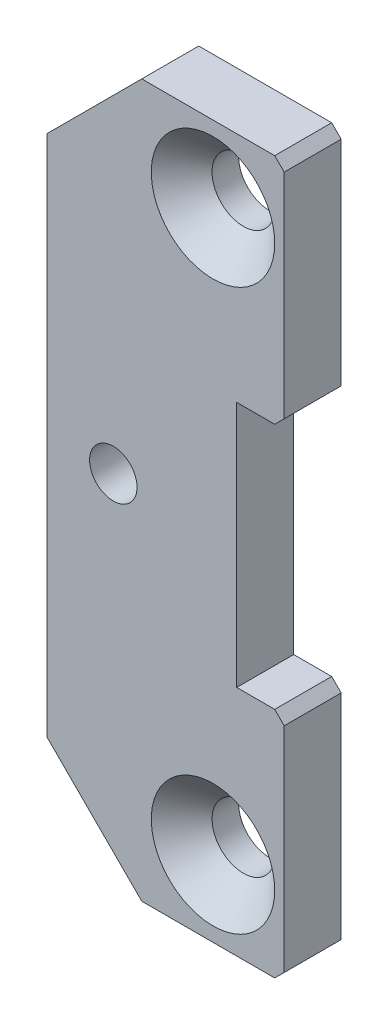
SolidWorks part; units mm, degrees
material "Q235-A"
ref_plane "Front Plane" through (0, 0, 0) normal (0, 0, 1) x (1, 0, 0)
ref_plane "Top Plane" through (0, 0, 0) normal (0, 1, 0) x (1, 0, 0)
ref_plane "Right Plane" through (0, 0, 0) normal (1, 0, 0) x (0, 0, -1)
sketch "Sketch1" plane through (0, 0, 0) normal (0, 0, 1) x (1, 0, 0)
  line L0 (0, 75) -> (0, 0)
  dimension "D2" = 75
extrude "Extrude-Thin1" add sketch "Sketch1" along normal blind 6 thin
chamfer "Chamfer1" distance 1 angle 45 2 edges at (0, 75, 3) (0, 0, 3)
hole_wizard "Hole size (per socket flat counteBLZKk head screw type)1" positions "Sketch7" profile "Sketch9" countersink size "M6" standard "GB" end condition through all
sketch "Sketch7" plane through (0, 0, 6) normal (0, 0, 1) x (1, 0, 0)
  line L1 (-25, 75) -> (-1, 75) construction
  line L4 (-25, 37.5) -> (0, 37.5) construction
  line L5 (-25, 75) -> (-25, 0) construction
  line L6 (0, 74) -> (0, 1) construction
  point P0 (-7.5, 67)
  point P2 (-7.5, 8)
  dimension "D1" = 8
  dimension "D2" = 7.5
sketch "Sketch9" plane through (-7.5, 67, 6) normal (1, 0, 0) x (0, -1, 0)
  line L0 (0, 0) -> (0, 6)
  line L1 (0, 6) -> (3.3, 6)
  line L2 (3.3, 6) -> (3.3, 3.2)
  line L3 (3.3, 3.2) -> (6.5, 0)
  line L5 (6.5, 0) -> (0, 0)
  line L6 (-3.3, 3.2) -> (-6.5, 0) construction
  line L11 (0, -6.35) -> (0, 107.95) construction
  dimension "通孔孔直径" = 6.6
  dimension "通孔孔深度" = 6
  dimension "近端锥形沉头孔直径" = 13
  dimension "近端锥形沉头孔角度" = 90
chamfer "Chamfer2" distance 10 angle 45 2 edges at (-25, 0, 3) (-25, 75, 3)
hole_wizard "M6 Tapped Hole1" positions "Sketch10" profile "Sketch11" tap size "M6" standard "GB" end condition through all
sketch "Sketch10" plane through (0, 0, 6) normal (0, 0, 1) x (1, 0, 0)
  line L0 (0, 37.5) -> (-51.0681, 37.5)
  line L1 (0, 74) -> (0, 1) construction
  line L3 (-25, 65) -> (-25, 10) construction
  point P0 (-18, 37.5)
  dimension "D1" = 7
sketch "Sketch11" plane through (-18, 37.5, 6) normal (1, 0, 0) x (0, -1, 0)
  line L0 (0, 0) -> (0, 6)
  line L1 (0, 6) -> (2.5, 6)
  line L2 (2.5, 6) -> (2.5, 0)
  line L5 (2.5, 0) -> (0, 0)
  line L11 (0, -6.35) -> (0, 107.95) construction
  dimension "通孔螺纹孔钻头直径" = 5
  dimension "通孔螺纹孔钻头深度" = 6
cosmetic thread "Cosmetic thread 1"
sketch "Sketch12" plane through (0, 0, 6) normal (0, 0, 1) x (1, 0, 0)
  line L0 (-25, 37.5) -> (35.2592, 37.5) construction
  line L1 (-25, 65) -> (-25, 10) construction
  line L2 (0, 74) -> (0, 1) construction
  line L3 (15.2592, 50.5) -> (-5, 50.5)
  line L4 (15.2592, 50.5) -> (15.2592, 24.5)
  line L5 (15.2592, 24.5) -> (-5, 24.5)
  line L6 (-5, 50.5) -> (-5, 24.5)
  line L7 (15.2592, 50.5) -> (-5, 24.5) construction
  line L8 (15.2592, 24.5) -> (-5, 50.5) construction
  point P4 (5.1296, 37.5)
  dimension "D1" = 26
  dimension "D2" = 5
extrude "Cut-Extrude1" cut sketch "Sketch12" against normal blind 10
chamfer "Chamfer3" distance 1 angle 45 2 edges at (0, 24.5, 3) (0, 50.5, 3)
